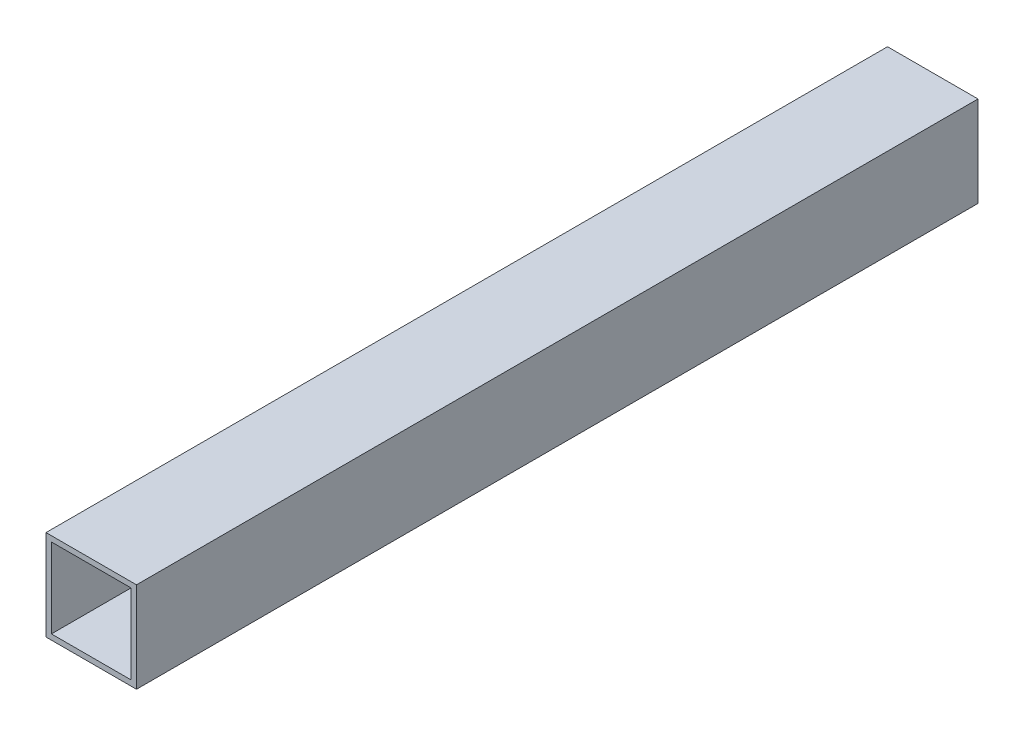
from build123d import *

# Parameters (mm, degrees)
SKETCH_1_W      = 50
SKETCH_1_H      = 50
SKETCH_1_W_2    = 44
SKETCH_1_H_2    = 44
EXTRUDE_1_DEPTH = 465


with BuildPart() as part:
    # 草图1 → 凸台-拉伸1 (new body)
    with BuildSketch(Plane.XY):
        with Locations((25, 25)):
            Rectangle(SKETCH_1_W, SKETCH_1_H)
        with Locations((25, 25)):
            Rectangle(SKETCH_1_W_2, SKETCH_1_H_2, mode=Mode.SUBTRACT)
    extrude(amount=EXTRUDE_1_DEPTH)


solid = part.part
